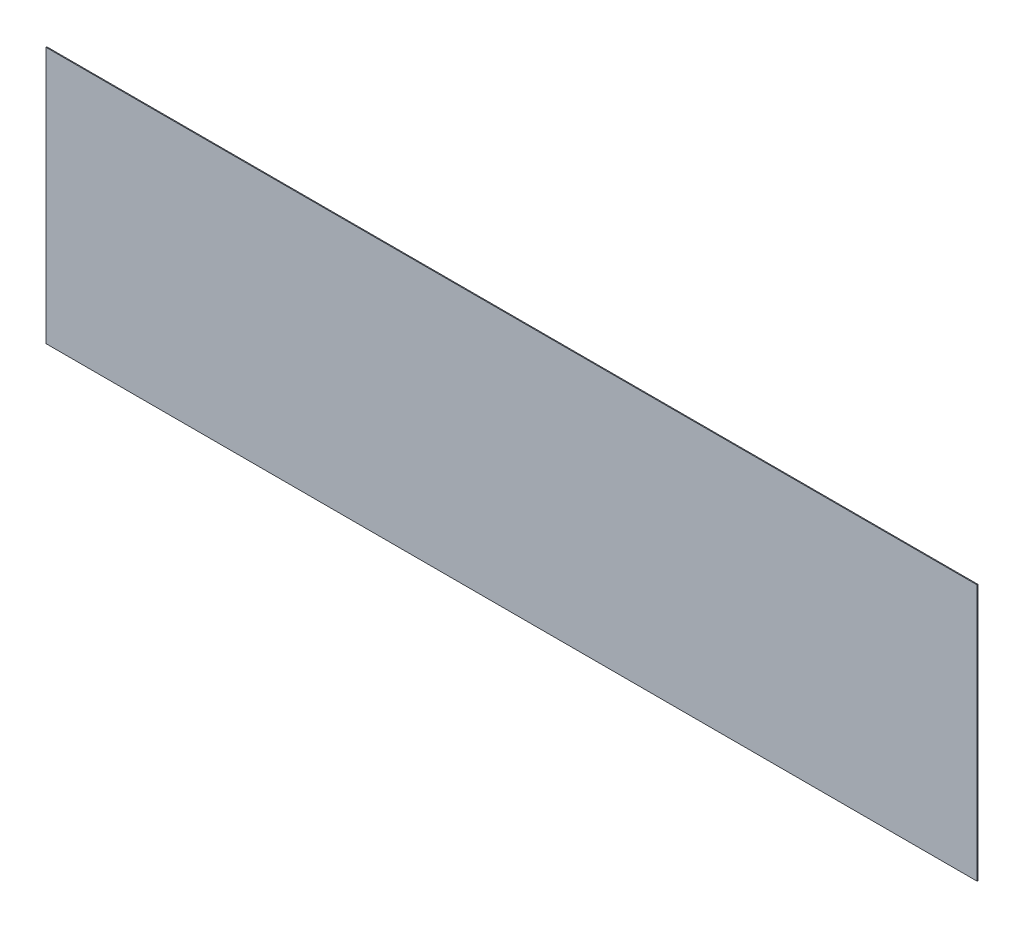
SolidWorks part; units mm, degrees
ref_plane "Front Plane" through (0, 0, 0) normal (0, 0, 1) x (1, 0, 0)
ref_plane "Top Plane" through (0, 0, 0) normal (0, 1, 0) x (1, 0, 0)
ref_plane "Right Plane" through (0, 0, 0) normal (1, 0, 0) x (0, 0, -1)
sketch "Sketch1" plane through (0, 0, 0) normal (0, 0, 1) x (1, 0, 0)
  line L1 (0, 0) -> (1560, 0)
  line L2 (0, 0) -> (0, 430)
  line L3 (0, 430) -> (1560, 430)
  line L4 (1560, 0) -> (1560, 430)
extrude "Boss-Extrude1" add sketch "Sketch1" along normal blind 1.5
